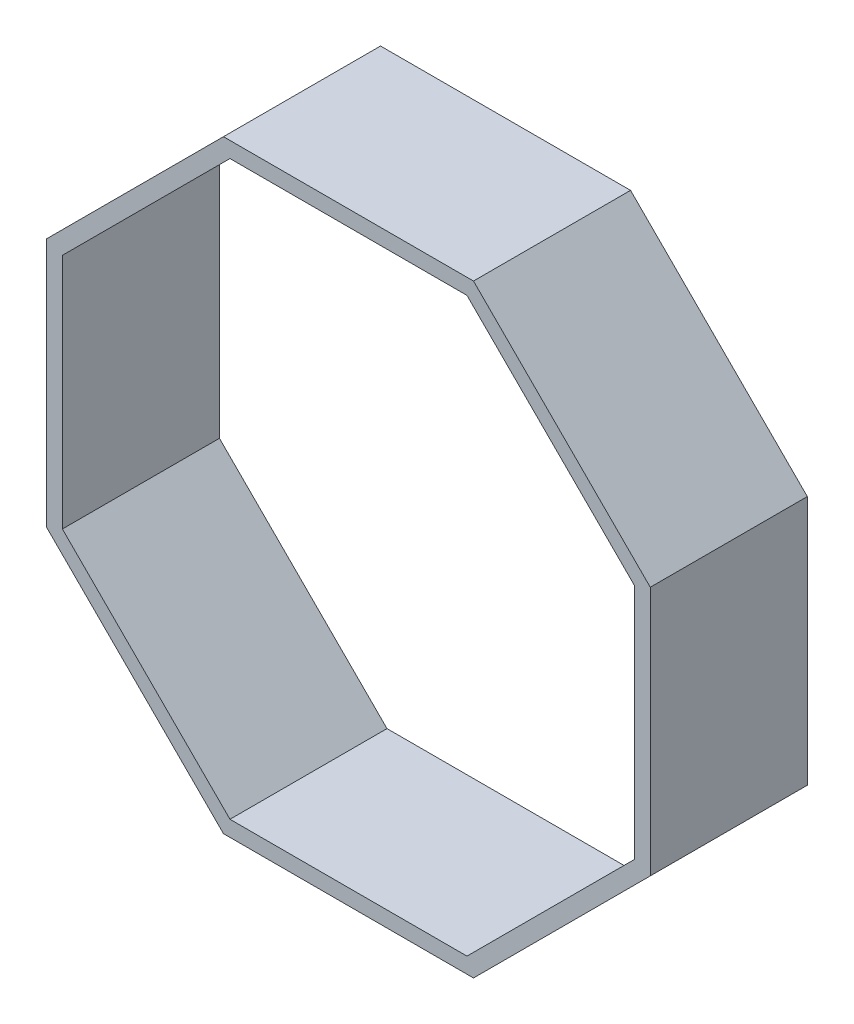
SolidWorks part; units mm, degrees
ref_plane "前视基准面" through (0, 0, 0) normal (0, 0, 1) x (1, 0, 0)
ref_plane "上视基准面" through (0, 0, 0) normal (0, 1, 0) x (1, 0, 0)
ref_plane "右视基准面" through (0, 0, 0) normal (1, 0, 0) x (0, 0, -1)
sketch "草图1" plane through (0, 0, 0) normal (0, 0, 1) x (1, 0, 0)
  line L7 (-39.7991, 96.0835) -> (-96.0835, 39.7991)
  line L8 (-96.0835, 39.7991) -> (-96.0835, -39.7991)
  line L9 (-96.0835, -39.7991) -> (-39.7991, -96.0835)
  line L10 (-39.7991, -96.0835) -> (39.7991, -96.0835)
  line L11 (39.7991, -96.0835) -> (96.0835, -39.7991)
  line L12 (96.0835, -39.7991) -> (96.0835, 39.7991)
  line L13 (96.0835, 39.7991) -> (39.7991, 96.0835)
  line L14 (39.7991, 96.0835) -> (-39.7991, 96.0835)
  circle A0 centre (0, 0) radius 96.0835 construction
  dimension "D1" = 208
extrude "凸台-拉伸1" add sketch "草图1" along normal blind 50
sketch "草图2" plane through (0, 0, 50) normal (0, 0, 1) x (1, 0, 0)
  line L8 (37.728, 91.0835) -> (-37.728, 91.0835)
  line L9 (37.728, 91.0835) -> (-37.728, 91.0835)
  line L10 (-37.728, 91.0835) -> (-91.0835, 37.728)
  line L11 (-37.728, 91.0835) -> (-91.0835, 37.728)
  line L12 (-91.0835, 37.728) -> (-91.0835, -37.728)
  line L13 (-91.0835, 37.728) -> (-91.0835, -37.728)
  line L14 (-91.0835, -37.728) -> (-37.728, -91.0835)
  line L15 (-91.0835, -37.728) -> (-37.728, -91.0835)
  line L16 (-37.728, -91.0835) -> (37.728, -91.0835)
  line L17 (-37.728, -91.0835) -> (37.728, -91.0835)
  line L24 (37.728, -91.0835) -> (91.0835, -37.728)
  line L25 (37.728, -91.0835) -> (91.0835, -37.728)
  line L26 (91.0835, -37.728) -> (91.0835, 37.728)
  line L27 (91.0835, -37.728) -> (91.0835, 37.728)
  line L28 (91.0835, 37.728) -> (37.728, 91.0835)
  line L29 (91.0835, 37.728) -> (37.728, 91.0835)
  dimension "D1" = 5
extrude "切除-拉伸1" cut sketch "草图2" against normal blind 606
sketch "草图3" plane through (0, 0, 50) normal (0, 0, 1) x (1, 0, 0)
  circle A0 centre (0, 0) radius 36.8451
